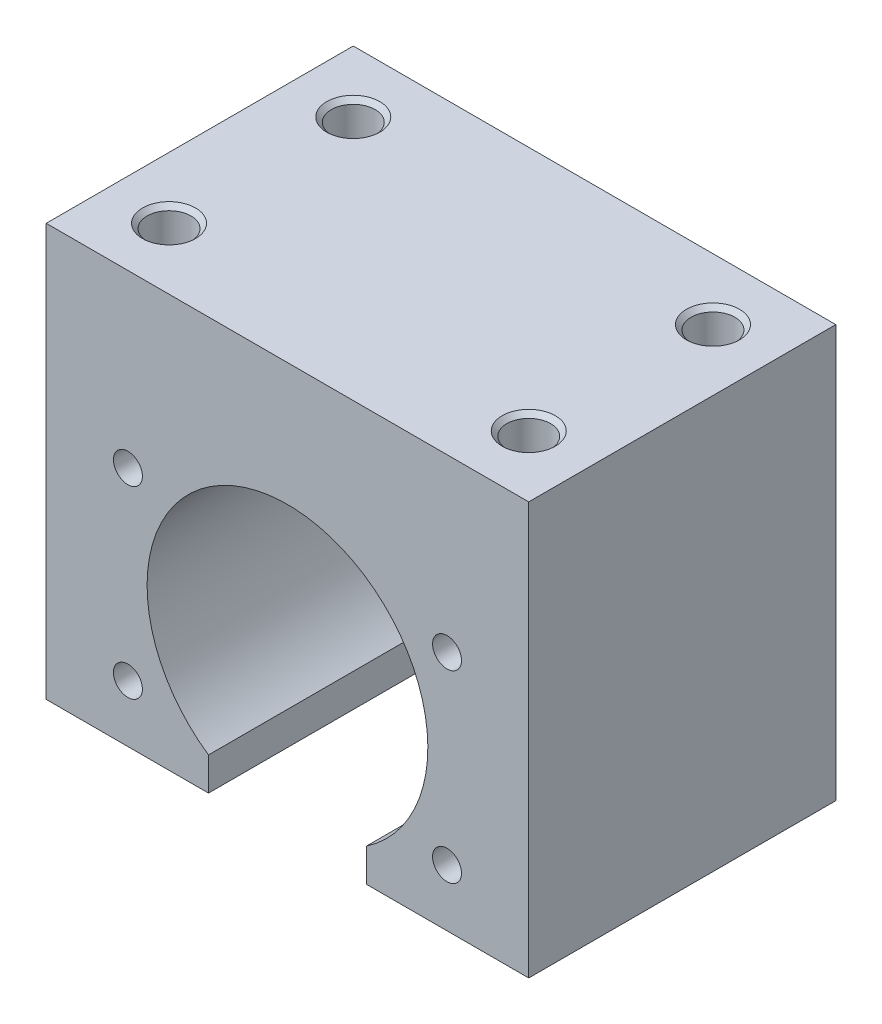
from build123d import *

# Parameters (mm, degrees)
EXTRUDE_1_DEPTH              = 17.5
HOLE_WIZARD_M4_1_D           = 3.3
HOLE_WIZARD_M4_1_DEPTH       = 9.5
HOLE_WIZARD_M4_1_TIP         = 0.991420021
HOLE_WIZARD_M6_1_D           = 5
HOLE_WIZARD_M6_1_DEPTH       = 12
HOLE_WIZARD_M6_1_CSINK_D     = 6.05
HOLE_WIZARD_M6_1_CSINK_ANGLE = 90
HOLE_WIZARD_M6_1_TIP         = 1.502151548


with BuildPart() as part:
    # 草图1 → 凸台-拉伸1 (new, symmetric)
    with BuildSketch(Plane.XY):
        with BuildLine():
            Line((-27.5, 30), (27.5, 30))
            Line((27.5, 30), (27.5, -17))
            Line((27.5, -17), (9, -17))
            Line((9, -17), (9, -13.228756555))
            ThreePointArc((9, -13.228756555), (0, 16), (-9, -13.228756555))
            Line((-9, -13.228756555), (-9, -17))
            Line((-9, -17), (-27.5, -17))
            Line((-27.5, -17), (-27.5, 30))
        make_face()
    extrude(amount=EXTRUDE_1_DEPTH, both=True)

    # M4 螺纹孔1
    with Locations(Plane.XY.offset(17.5)):
        with Locations((18.186533479, 10.5), (18.186533479, -10.5), (-18.186533479, -10.5), (-18.186533479, 10.5)):
            Hole(HOLE_WIZARD_M4_1_D / 2, depth=HOLE_WIZARD_M4_1_DEPTH)
            with Locations((0, 0, -(HOLE_WIZARD_M4_1_DEPTH + HOLE_WIZARD_M4_1_TIP / 2))):  # 118° drill point
                Cone(0, HOLE_WIZARD_M4_1_D / 2, HOLE_WIZARD_M4_1_TIP, mode=Mode.SUBTRACT)

    # M6 螺纹孔1
    with Locations(Plane(origin=(-20.5, 30, 10.5), x_dir=(0, 0, 1), z_dir=(0, 1, 0))):
        with Locations((0, 0), (-21, 0), (-21, 41), (0, 41)):
            CounterSinkHole(HOLE_WIZARD_M6_1_D / 2, HOLE_WIZARD_M6_1_CSINK_D / 2, depth=HOLE_WIZARD_M6_1_DEPTH, counter_sink_angle=HOLE_WIZARD_M6_1_CSINK_ANGLE)
            with Locations((0, 0, -(HOLE_WIZARD_M6_1_DEPTH + HOLE_WIZARD_M6_1_TIP / 2))):  # 118° drill point
                Cone(0, HOLE_WIZARD_M6_1_D / 2, HOLE_WIZARD_M6_1_TIP, mode=Mode.SUBTRACT)


solid = part.part
